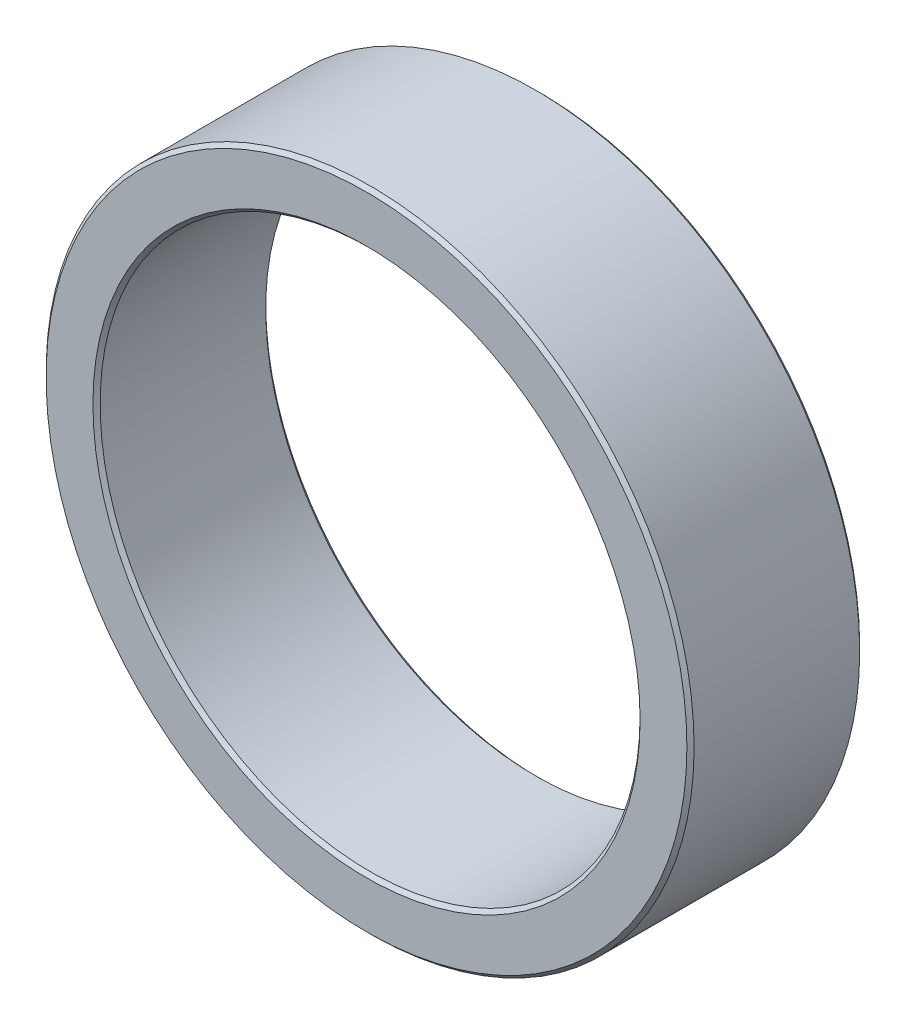
from build123d import *

# Parameters (mm, degrees)
SKETCH1_R           = 45
SKETCH1_R_2         = 37.5
BOSS_EXTRUDE1_DEPTH = 24
CHAMFER1_SIZE       = 0.5


with BuildPart() as part:
    # Sketch1 → Boss-Extrude1 (new body)
    with BuildSketch(Plane.XY):
        Circle(SKETCH1_R)
        Circle(SKETCH1_R_2, mode=Mode.SUBTRACT)
    extrude(amount=BOSS_EXTRUDE1_DEPTH)

    # Chamfer1
    chamfer1_edges = [part.edges().sort_by_distance(p)[0] for p in [
        (-45, 0, 0),
        (-45, 0, 24),
        (-37.5, 0, 0),
        (-37.5, 0, 24),
    ]]
    chamfer(chamfer1_edges, length=CHAMFER1_SIZE)


solid = part.part
